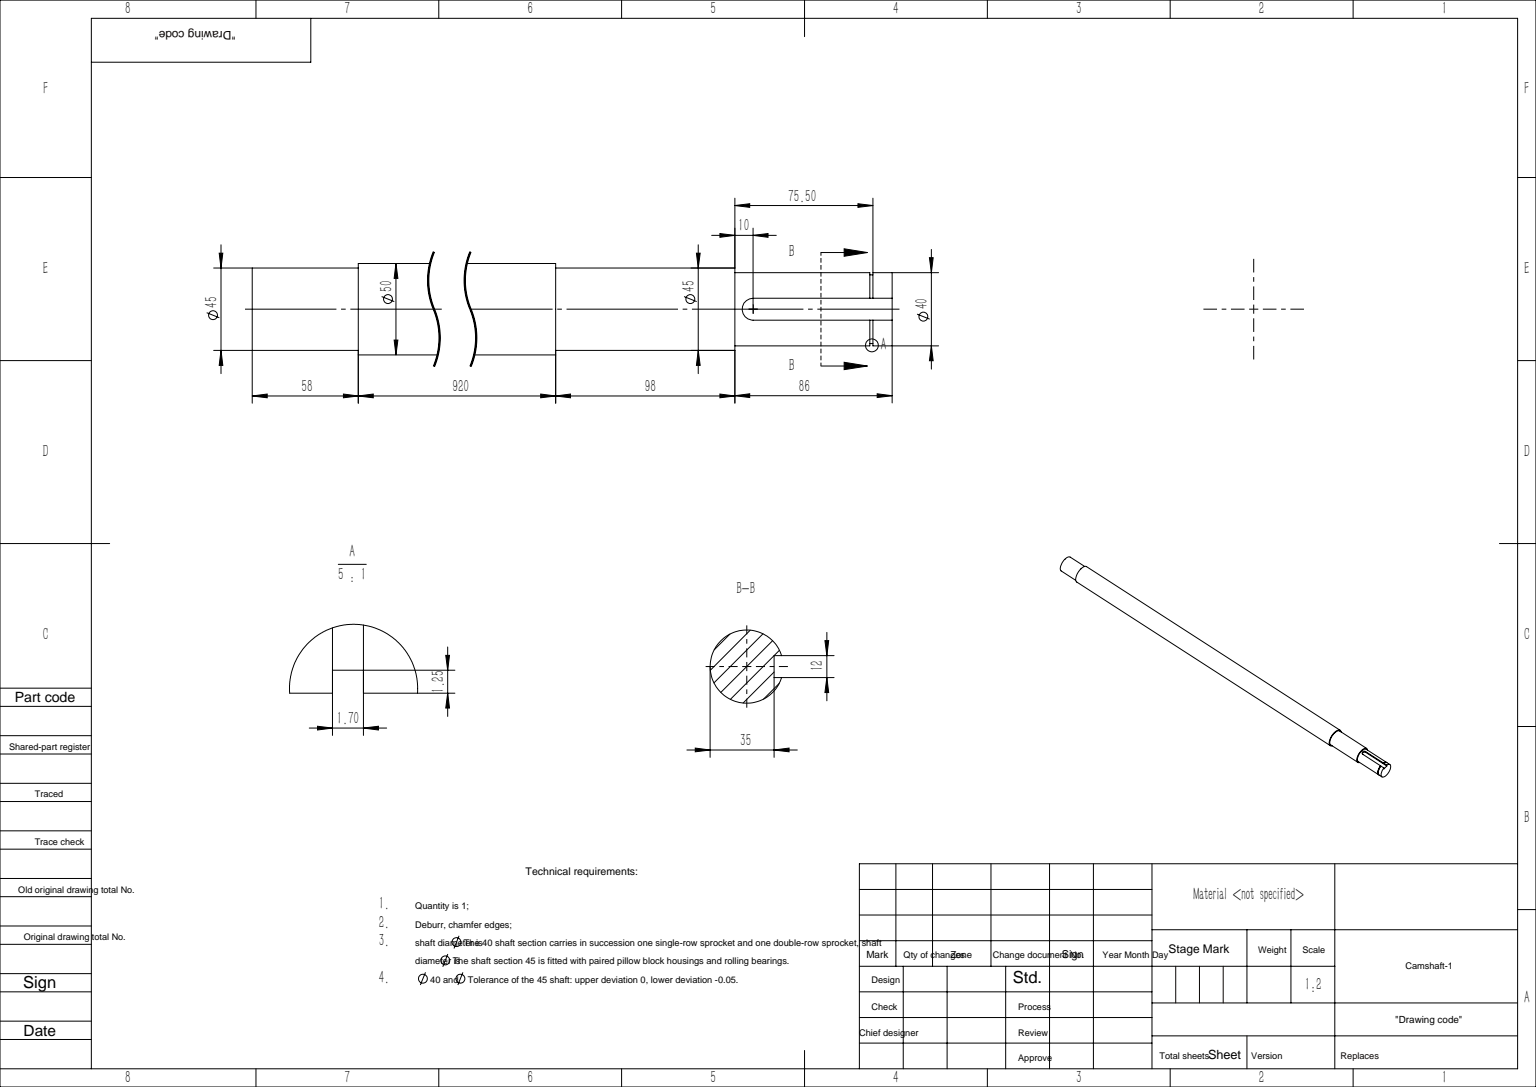
SolidWorks part; units mm, degrees
ref_plane "前视基准面" through (0, 0, 0) normal (0, 0, 1) x (1, 0, 0)
ref_plane "上视基准面" through (0, 0, 0) normal (0, 1, 0) x (1, 0, 0)
ref_plane "右视基准面" through (0, 0, 0) normal (1, 0, 0) x (0, 0, -1)
sketch "草图1" plane through (0, 0, 0) normal (0, 0, 1) x (1, 0, 0)
  line L0 (0, 0) -> (0, 22.5)
  line L1 (0, 22.5) -> (58, 22.5)
  line L2 (58, 22.5) -> (58, 25)
  line L3 (58, 25) -> (978, 25)
  line L4 (978, 25) -> (978, 22.5)
  line L5 (978, 22.5) -> (1076, 22.5)
  line L6 (1076, 22.5) -> (1076, 20)
  line L7 (1076, 20) -> (1162, 20)
  line L8 (1162, 20) -> (1162, 0)
  line L9 (1162, 0) -> (0, 0)
  dimension "D1" = 58
  dimension "D2" = 920
  dimension "D3" = 98
  dimension "D4" = 86
  dimension "D5" = 25
  dimension "D6" = 22.5
  dimension "D7" = 22.5
  dimension "D8" = 20
revolve "旋转1" add sketch "草图1" angle 360 about L9
ref_plane "基准面1" through (0, 20, 0) normal (0, 1, 0) x (1, 0, 0)
sketch "草图2" plane through (0, 20, 0) normal (0, 1, 0) x (1, 0, 0)
  line L0 (1076, 0) -> (1162, 0) construction
  line L3 (1076, -22.5) -> (1076, 22.5) construction
  line L4 (1162, -20) -> (1162, 20) construction
  line L5 (1076, -20) -> (1076, 20) construction
  line L6 (1086, 6) -> (1172, 6)
  line L7 (1172, 6) -> (1172, -6)
  line L8 (1172, -6) -> (1086, -6)
  arc A0 (1086, 6) -> (1086, -6) centre (1086, 0) ccw
  dimension "D1" = 12
  dimension "D3" = 10
  dimension "D2" = 10
extrude "切除-拉伸1" cut sketch "草图2" against normal blind 5
ref_plane "基准面2" through (1151.5, 0, 0) normal (1, 0, 0) x (0, 0, -1)
sketch "草图3" plane through (1151.5, 0, 0) normal (1, 0, 0) x (0, 0, -1)
  circle A0 centre (0, 0) radius 18.75
  circle A1 centre (0, 0) radius 20
  arc A2 (-6, 19.0788) -> (6, 19.0788) centre (0, 0) ccw construction
  dimension "D2" = 37.5
extrude "切除-拉伸2" cut sketch "草图3" against normal blind 1.7
